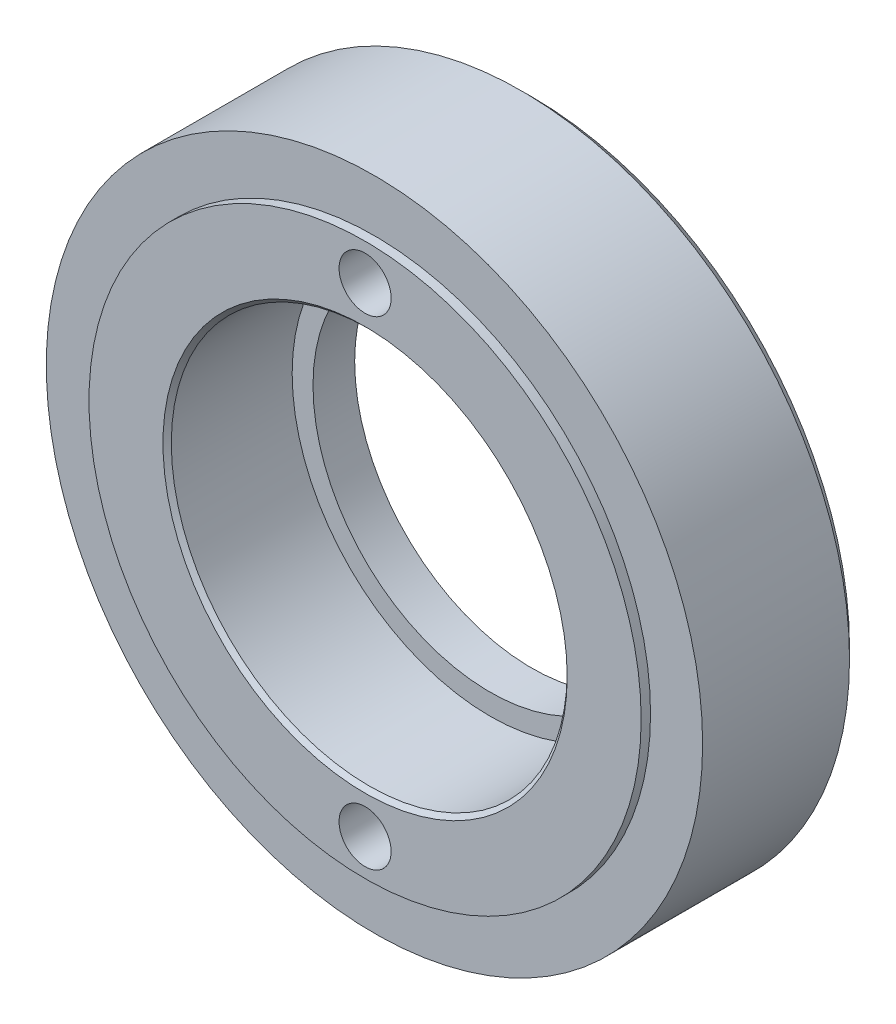
from build123d import *

# Parameters (mm, degrees)
SKETCH1_R           = 15.75
SKETCH1_R_2         = 9.5
BOSS_EXTRUDE1_DEPTH = 4
SKETCH3_R           = 10.639095477
SKETCH3_R_2         = 8.5
BOSS_EXTRUDE2_DEPTH = 2
M3_TAPPED_HOLE1_D   = 2.5
CHAMFER1_SIZE       = 0.2
SKETCH6_R           = 20.677002962
SKETCH6_R_2         = 13.25
CUT_EXTRUDE1_DEPTH  = 0.45
CHAMFER2_SIZE       = 0.5


with BuildPart() as part:
    # Sketch1 → Boss-Extrude1 (new, symmetric)
    with BuildSketch(Plane.XY):
        Circle(SKETCH1_R)
        Circle(SKETCH1_R_2, mode=Mode.SUBTRACT)
    extrude(amount=BOSS_EXTRUDE1_DEPTH, both=True)

    # Sketch3 → Boss-Extrude2 (add)
    with BuildSketch(Plane(origin=(0, 0, -4), x_dir=(-1, 0, 0), z_dir=(0, 0, -1))):
        Circle(SKETCH3_R)
        Circle(SKETCH3_R_2, mode=Mode.SUBTRACT)
    extrude(amount=-BOSS_EXTRUDE2_DEPTH)

    # M3 Tapped Hole1 (through all)
    with Locations(Plane.XY.offset(4)):
        with Locations((0, -11.5)):
            m3_tapped_hole1 = Hole(M3_TAPPED_HOLE1_D / 2)

    # Mirror1: M3 Tapped Hole1 across plane
    add(m3_tapped_hole1.mirror(Plane.ZX), mode=Mode.SUBTRACT)

    # Chamfer1
    chamfer1_edges = [part.edges().sort_by_distance(p)[0] for p in [
        (-9.5, 0, 4),
    ]]
    chamfer(chamfer1_edges, length=CHAMFER1_SIZE)

    # Sketch6 → Cut-Extrude1 (cut)
    with BuildSketch(Plane.XY.offset(4)):
        Circle(SKETCH6_R)
        Circle(SKETCH6_R_2, mode=Mode.SUBTRACT)
    extrude(amount=-CUT_EXTRUDE1_DEPTH, mode=Mode.SUBTRACT)

    # Chamfer2
    chamfer2_edges = [part.edges().sort_by_distance(p)[0] for p in [
        (-15.75, 0, -4),
    ]]
    chamfer(chamfer2_edges, length=CHAMFER2_SIZE)


solid = part.part
